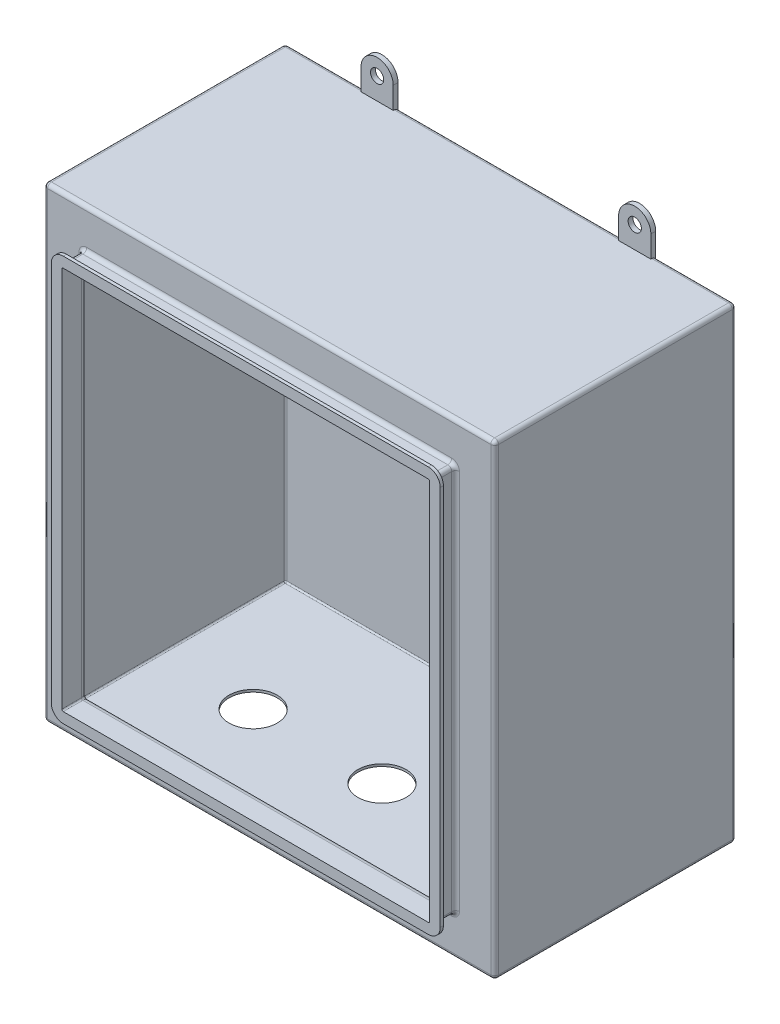
from build123d import *

# Parameters (mm, degrees)
SKETCH_1_W          = 280
SKETCH_1_H          = 150
EXTRUDE_1_DEPTH     = 290
FILLET_1_R          = 2.4
SKETCH_2_W          = 231.48
SKETCH_2_H          = 241.48
EXTRUDE_2_DEPTH     = 14.57
FILLET_2_R          = 2.4
SHELL_1_T           = -1.5
SKETCH_3_R          = 15
CUT_EXTRUDE_1_DEPTH = 333.948997446
SKETCH_4_R          = 4.1
EXTRUDE_3_DEPTH     = 3
EXTRUDE_4_DEPTH     = 2


with BuildPart() as part:
    # 草图1 → 凸台-拉伸1 (new body)
    with BuildSketch(Plane(origin=(0, 0, 0), x_dir=(1, 0, 0), z_dir=(0, 1, 0))):
        Rectangle(SKETCH_1_W, SKETCH_1_H)
    extrude(amount=EXTRUDE_1_DEPTH)

    # 圆角1
    fillet_1_edges = [part.edges().sort_by_distance(p)[0] for p in [
        (-140, 290, 0),
        (0, 290, 75),
        (140, 290, 0),
        (0, 0, 75),
        (-140, 0, 0),
        (0, 0, -75),
        (140, 0, 0),
        (0, 290, -75),
        (140, 145, 75),
        (-140, 145, 75),
        (-140, 145, -75),
        (140, 145, -75),
    ]]
    fillet(fillet_1_edges, radius=FILLET_1_R)

    # 草图2 → 凸台-拉伸2 (add)
    with BuildSketch(Plane.XY.offset(75)):
        with Locations((0, 145)):
            Rectangle(SKETCH_2_W, SKETCH_2_H)
    extrude(amount=EXTRUDE_2_DEPTH)

    # 圆角2
    fillet_2_edges = [part.edges().sort_by_distance(p)[0] for p in [
        (-115.74, 145, 75),
        (-115.74, 265.74, 82.285),
        (0, 24.26, 75),
        (-115.74, 24.26, 82.285),
        (115.74, 145, 75),
        (115.74, 24.26, 82.285),
        (0, 265.74, 75),
        (115.74, 265.74, 82.285),
    ]]
    fillet(fillet_2_edges, radius=FILLET_2_R)

    # 抽壳1
    shell_1_openings = [part.faces().sort_by_distance(p)[0] for p in [
        (0, 145, 89.57),
    ]]
    offset(amount=SHELL_1_T, openings=shell_1_openings, kind=Kind.INTERSECTION)

    # 草图3 → 切除-拉伸1 (cut, through all)
    with BuildSketch(Plane(origin=(0, 1.5, 0), x_dir=(1, 0, 0), z_dir=(0, 1, 0))):
        with Locations(Location((-80, -5, 0), (0, 0, 270))):
            Circle(SKETCH_3_R)
        with Locations(Location((0, -5, 0), (0, 0, 270))):
            Circle(SKETCH_3_R)
        with Locations(Location((80, -5, 0), (0, 0, 270))):
            Circle(SKETCH_3_R)
    extrude(amount=-CUT_EXTRUDE_1_DEPTH, mode=Mode.SUBTRACT)

    # 草图4 → 凸台-拉伸3 (add)
    # profile 1 of 4: a face of its own
    with BuildSketch(Plane(origin=(0, 0, -75), x_dir=(-1, 0, 0), z_dir=(0, 0, -1))):
        with BuildLine():
            Line((-90, 288.5), (-70, 288.5))
            Line((-70, 288.5), (-70, 303.5))
            ThreePointArc((-70, 303.5), (-80, 313.5), (-90, 303.5))
            Line((-90, 303.5), (-90, 288.5))
        make_face()
        with Locations(Location((-80, 303.5, 0), (0, 0, 180))):
            Circle(SKETCH_4_R, mode=Mode.SUBTRACT)
    # profile 2 of 4: a face of its own
    with BuildSketch(Plane(origin=(0, 0, -75), x_dir=(-1, 0, 0), z_dir=(0, 0, -1))):
        with BuildLine():
            Line((-90, 1.5), (-90, -13.5))
            ThreePointArc((-90, -13.5), (-80, -23.5), (-70, -13.5))
            Line((-70, -13.5), (-70, 1.5))
            Line((-70, 1.5), (-90, 1.5))
        make_face()
        with Locations((-80, -13.5)):
            Circle(SKETCH_4_R, mode=Mode.SUBTRACT)
    # profile 3 of 4: a face of its own
    with BuildSketch(Plane(origin=(0, 0, -75), x_dir=(-1, 0, 0), z_dir=(0, 0, -1))):
        with BuildLine():
            Line((70, 1.5), (70, -13.5))
            ThreePointArc((70, -13.5), (80, -23.5), (90, -13.5))
            Line((90, -13.5), (90, 1.5))
            Line((90, 1.5), (70, 1.5))
        make_face()
        with Locations((80, -13.5)):
            Circle(SKETCH_4_R, mode=Mode.SUBTRACT)
    # profile 4 of 4: a face of its own
    with BuildSketch(Plane(origin=(0, 0, -75), x_dir=(-1, 0, 0), z_dir=(0, 0, -1))):
        with BuildLine():
            Line((70, 288.5), (90, 288.5))
            Line((90, 288.5), (90, 303.5))
            ThreePointArc((90, 303.5), (80, 313.5), (70, 303.5))
            Line((70, 303.5), (70, 288.5))
        make_face()
        with Locations(Location((80, 303.5, 0), (0, 0, 180))):
            Circle(SKETCH_4_R, mode=Mode.SUBTRACT)
    extrude(amount=-EXTRUDE_3_DEPTH)

    # 草图5 → 凸台-拉伸4 (add)
    with BuildSketch(Plane.XY.offset(89.57)):
        with BuildLine():
            Line((-120.74, 263.34), (-120.74, 26.66))
            ThreePointArc((-120.74, 26.66), (-118.572590181, 21.427409819), (-113.34, 19.26))
            Line((-113.34, 19.26), (113.34, 19.26))
            ThreePointArc((113.34, 19.26), (118.572590181, 21.427409819), (120.74, 26.66))
            Line((120.74, 26.66), (120.74, 263.34))
            ThreePointArc((120.74, 263.34), (118.572590181, 268.572590181), (113.34, 270.74))
            Line((113.34, 270.74), (-113.34, 270.74))
            ThreePointArc((-113.34, 270.74), (-118.572590181, 268.572590181), (-120.74, 263.34))
        make_face()
        with BuildLine():
            Line((-115.74, 263.34), (-115.74, 26.66))
            ThreePointArc((-115.74, 26.66), (-115.037056275, 24.962943725), (-113.34, 24.26))
            Line((-113.34, 24.26), (113.34, 24.26))
            ThreePointArc((113.34, 24.26), (115.037056275, 24.962943725), (115.74, 26.66))
            Line((115.74, 26.66), (115.74, 263.34))
            ThreePointArc((115.74, 263.34), (115.037056275, 265.037056275), (113.34, 265.74))
            Line((113.34, 265.74), (-113.34, 265.74))
            ThreePointArc((-113.34, 265.74), (-115.037056275, 265.037056275), (-115.74, 263.34))
        make_face(mode=Mode.SUBTRACT)
    extrude(amount=-EXTRUDE_4_DEPTH)


solid = part.part
